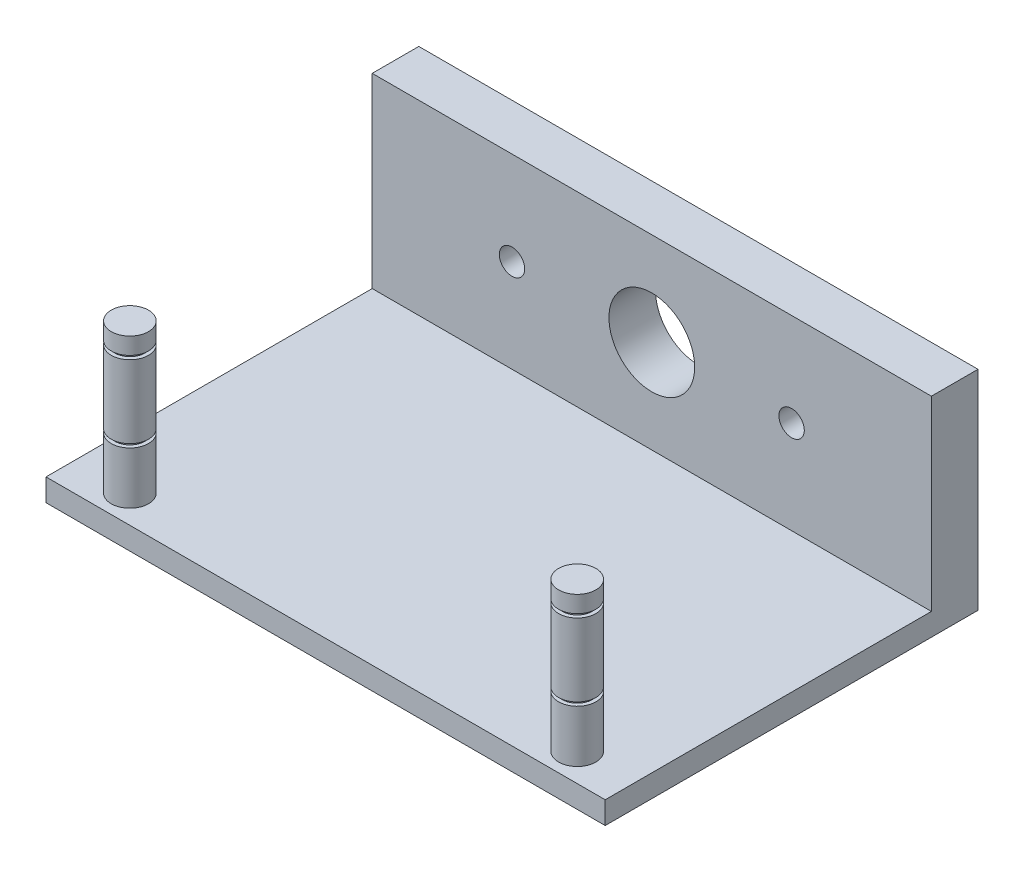
SolidWorks part; units mm, degrees
ref_plane "Front Plane" through (0, 0, 0) normal (0, 0, 1) x (1, 0, 0)
ref_plane "Top Plane" through (0, 0, 0) normal (0, 1, 0) x (1, 0, 0)
ref_plane "Right Plane" through (0, 0, 0) normal (1, 0, 0) x (0, 0, -1)
sketch "Sketch1" plane through (0, 0, 0) normal (0, 0, 1) x (1, 0, 0)
  line L1 (-100, -25) -> (100, -25)
  line L2 (-100, -25) -> (-100, 25)
  line L3 (-100, 25) -> (100, 25)
  line L4 (100, -25) -> (100, 25)
  line L5 (-100, -25) -> (100, 25) construction
  line L6 (-100, 25) -> (100, -25) construction
  circle A0 centre (0, 0) radius 11.5
  point P0 (0, 0)
  dimension "D3" = 23
  dimension "D1" = 50
  dimension "D2" = 200
extrude "Boss-Extrude1" add sketch "Sketch1" along normal blind 12.5
sketch "Sketch2" plane through (0, -25, 0) normal (0, -1, 0) x (1, 0, 0)
  line L1 (-100, 0) -> (100, 0)
  line L2 (-100, 0) -> (-100, 100)
  line L3 (-100, 100) -> (100, 100)
  line L4 (100, 0) -> (100, 100)
  dimension "D1" = 200
  dimension "D2" = 100
extrude "Boss-Extrude2" add sketch "Sketch2" along normal blind 6
sketch "Sketch3" plane through (0, 0, 0) normal (0, 0, -1) x (-1, 0, 0)
  line L0 (0, 0) -> (-37.5, 0) construction
  line L1 (0, 0) -> (37.5, 0) construction
  dimension "D1" = 37.5
  dimension "D2" = 37.5
hole_wizard "M8x1.25 Tapped Hole1" positions "3DSketch2" profile "Sketch5" tap size "M8x1.25" standard "Ansi Metric"
sketch3d "3DSketch2"
  point P0 (37.5, 0, 0)
  point P3 (-37.5, 0, 0)
sketch "Sketch5" plane through (37.5, 0, 0) normal (1, 0, 0) x (0, 1, 0)
  line L0 (0, 0) -> (0, 21.7929)
  line L1 (0, 21.7929) -> (3.4, 19.75)
  line L2 (3.4, 19.75) -> (3.4, 0)
  line L5 (3.4, 0) -> (0, 0)
  line L10 (0, 21.7929) -> (-3.4, 19.75) construction
  line L11 (0, -6.35) -> (0, 107.95) construction
  dimension "螺纹孔钻头直径" = 6.8
  dimension "螺纹孔钻头深度" = 19.75
  dimension "导头角度" = 118
cosmetic thread "Cosmetic Thread3" parameters "D1"=10, "D2"=8
cosmetic thread "Cosmetic Thread4" parameters "D1"=10, "D2"=8
sketch "Sketch6" plane through (0, -25, 0) normal (0, 1, 0) x (1, 0, 0)
  line L0 (-100, -12.5) -> (100, -12.5) construction
  circle A0 centre (60, -92.5) radius 5
  circle A1 centre (-60, -92.5) radius 5
  dimension "D5" = 10
  dimension "D6" = 10
  dimension "D1" = 60
  dimension "D2" = 60
  dimension "D3" = 80
  dimension "D4" = 80
extrude "Boss-Extrude3" add sketch "Sketch6" along normal blind 40
ref_plane "Plane1" through (0, 10.5, 0) normal (0, 1, 0) x (1, 0, 0)
sketch "Sketch7" plane through (0, 10.5, 0) normal (0, 1, 0) x (1, 0, 0)
  circle A0 centre (60, -92.5) radius 7.4083
  circle A1 centre (60, -92.5) radius 4
  circle A2 centre (-60, -92.5) radius 9.4736
  circle A3 centre (-60, -92.5) radius 4
  dimension "D1" = 8
  dimension "D2" = 8
extrude "Cut-Extrude1" cut sketch "Sketch7" against normal blind 1
ref_plane "Plane2" through (0, -10, 0) normal (0, 1, 0) x (1, 0, 0)
sketch "Sketch8" plane through (0, -10, 0) normal (0, 1, 0) x (1, 0, 0)
  circle A0 centre (60, -92.5) radius 11.6352
  circle A1 centre (60, -92.5) radius 4
  circle A2 centre (-60, -92.5) radius 12.8536
  circle A3 centre (-60, -92.5) radius 4
  dimension "D1" = 8
  dimension "D2" = 8
extrude "Cut-Extrude2" cut sketch "Sketch8" against normal blind 1
sketch "Sketch9" plane through (0, -31, 0) normal (0, -1, 0) x (1, 0, 0)
  line L0 (100, 0) -> (100, 100) construction
  line L1 (100, 0) -> (75, 0)
  line L2 (100, 0) -> (100, 100)
  line L3 (100, 100) -> (75, 100)
  line L4 (75, 0) -> (75, 100)
  line L5 (-100, 0) -> (100, 0) construction
  line L6 (100, 100) -> (-100, 100) construction
  line L7 (-100, 100) -> (-100, 0) construction
  line L8 (-100, 0) -> (-75, 0)
  line L9 (-100, 0) -> (-100, 100)
  line L10 (-100, 100) -> (-75, 100)
  line L11 (-75, 0) -> (-75, 100)
  dimension "D1" = 25
  dimension "D2" = 25
extrude "Cut-Extrude3" cut sketch "Sketch9" against normal up to next
